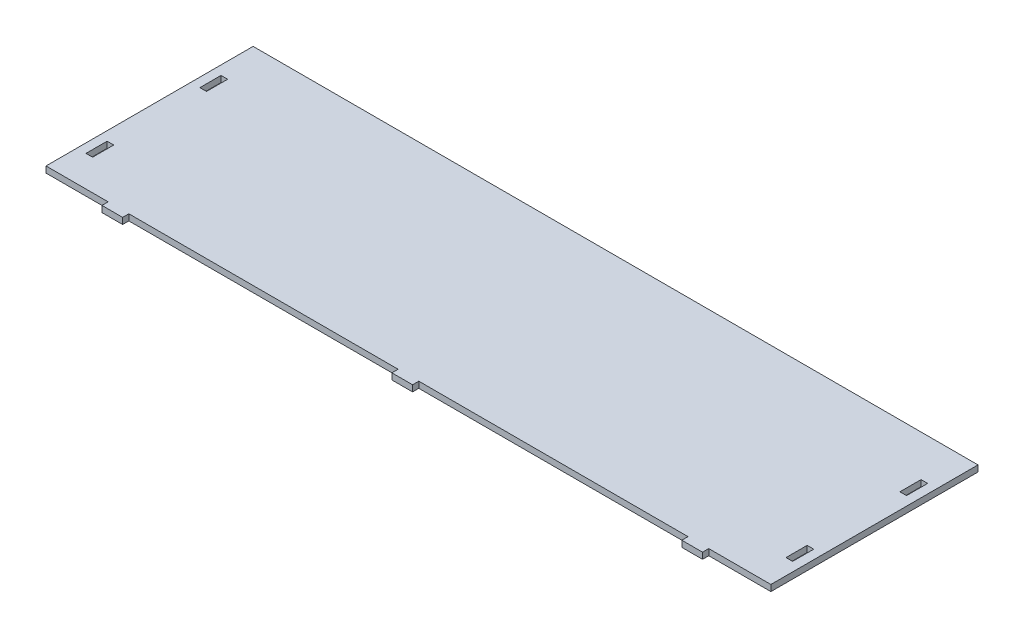
SolidWorks part; units mm, degrees
ref_plane "Front Plane" through (0, 0, 0) normal (0, 0, 1) x (1, 0, 0)
ref_plane "Top Plane" through (0, 0, 0) normal (0, 1, 0) x (1, 0, 0)
ref_plane "Right Plane" through (0, 0, 0) normal (1, 0, 0) x (0, 0, -1)
sketch "Sketch1" plane through (0, 0, 0) normal (0, 1, 0) x (1, 0, 0)
  line L1 (-175, -50) -> (175, -50)
  line L2 (-175, -50) -> (-175, 50)
  line L3 (-175, 50) -> (175, 50)
  line L4 (175, -50) -> (175, 50)
  line L5 (-175, -50) -> (175, 50) construction
  line L6 (-175, 50) -> (175, -50) construction
  point P0 (0, 0)
  dimension "D1" = 100
  dimension "D2" = 350
extrude "Boss-Extrude1" add sketch "Sketch1" along normal blind 3
sketch "Sketch2" plane through (0, 3, 0) normal (0, 1, 0) x (1, 0, 0)
  line L0 (175, 50) -> (-175, 50) construction
  line L1 (-170.6, 30.1) -> (-167.4, 30.1)
  line L2 (-170.6, 30.1) -> (-170.6, 19.9)
  line L3 (-170.6, 19.9) -> (-167.4, 19.9)
  line L4 (-167.4, 30.1) -> (-167.4, 19.9)
  line L5 (-170.6, -24.9) -> (-167.4, -24.9)
  line L6 (-170.6, -24.9) -> (-170.6, -35.1)
  line L7 (-170.6, -35.1) -> (-167.4, -35.1)
  line L8 (-167.4, -24.9) -> (-167.4, -35.1)
  line L9 (-175, -50) -> (175, -50) construction
  line L10 (-175, 50) -> (-175, -50) construction
  line L11 (0, -1000) -> (0, 49000) construction
  line L12 (167.4, -24.9) -> (167.4, -35.1)
  line L13 (170.6, -35.1) -> (167.4, -35.1)
  line L14 (170.6, -24.9) -> (170.6, -35.1)
  line L15 (170.6, -24.9) -> (167.4, -24.9)
  line L16 (167.4, 30.1) -> (167.4, 19.9)
  line L17 (170.6, 19.9) -> (167.4, 19.9)
  line L18 (170.6, 30.1) -> (170.6, 19.9)
  line L19 (170.6, 30.1) -> (167.4, 30.1)
  dimension "D1" = 10.2
  dimension "D2" = 3.2
  dimension "D3" = 19.9
  dimension "D4" = 14.9
  dimension "D5" = 10.2
  dimension "D6" = 3.2
  dimension "D7" = 4.4
  dimension "D8" = 4.4
extrude "Cut-Extrude1" cut sketch "Sketch2" against normal through all
sketch "Sketch3" plane through (0, 3, 0) normal (0, 1, 0) x (1, 0, 0)
  line L0 (-175, -50) -> (175, -50) construction
  line L1 (-145, -50) -> (-135, -50)
  line L2 (-145, -50) -> (-145, -53)
  line L3 (-145, -53) -> (-135, -53)
  line L4 (-135, -50) -> (-135, -53)
  line L5 (-175, 50) -> (-175, -50) construction
  line L10 (-5, -53) -> (5, -53)
  line L11 (-5, -53) -> (-5, -50)
  line L12 (-5, -50) -> (5, -50)
  line L13 (5, -53) -> (5, -50)
  line L14 (-5, -53) -> (5, -50) construction
  line L15 (-5, -50) -> (5, -53) construction
  line L16 (135, -50) -> (145, -50)
  line L17 (135, -50) -> (135, -53)
  line L18 (135, -53) -> (145, -53)
  line L19 (145, -50) -> (145, -53)
  line L20 (175, -50) -> (175, 50) construction
  point P6 (0, -51.5)
  dimension "D1" = 10
  dimension "D2" = 3
  dimension "D3" = 30
  dimension "D4" = 10
  dimension "D5" = 3
  dimension "D6" = 0
  dimension "D7" = 10
  dimension "D8" = 3
  dimension "D9" = 30
extrude "Boss-Extrude2" add sketch "Sketch3" against normal up to surface (3 mm away) up to face at (169, 0, -25)
